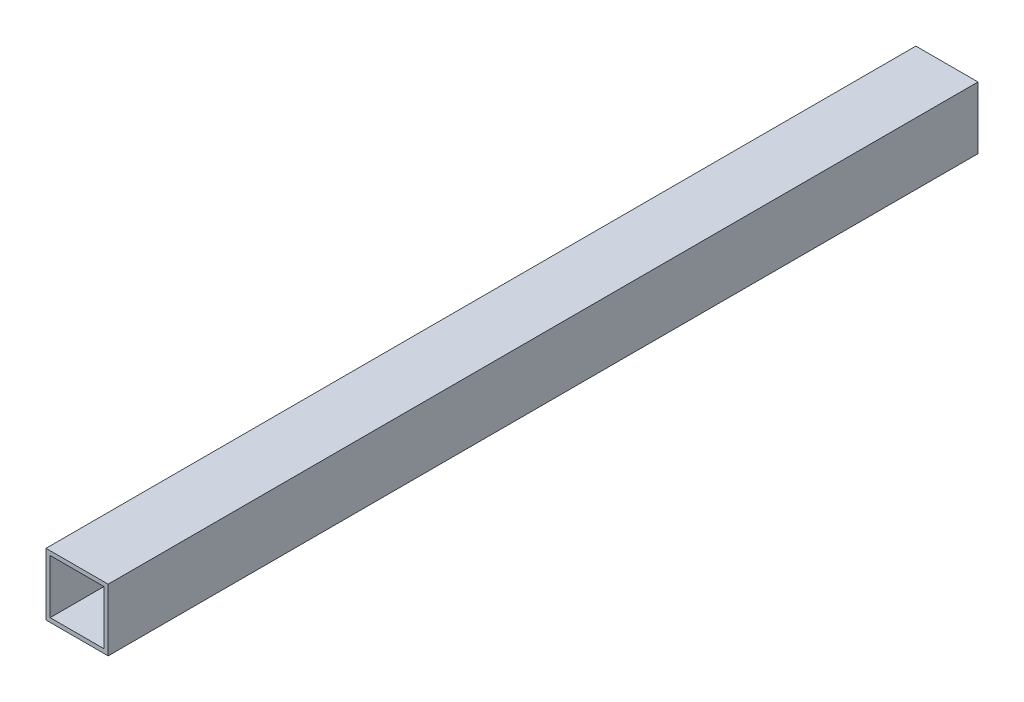
from build123d import *

# Parameters (mm, degrees)
SKETCH_1_W      = 30
SKETCH_1_H      = 30
SKETCH_1_W_2    = 26
SKETCH_1_H_2    = 26
EXTRUDE_1_DEPTH = 210


with BuildPart() as part:
    # 草图1 → 凸台-拉伸1 (new, symmetric)
    with BuildSketch(Plane.XY):
        Rectangle(SKETCH_1_W, SKETCH_1_H)
        Rectangle(SKETCH_1_W_2, SKETCH_1_H_2, mode=Mode.SUBTRACT)
    extrude(amount=EXTRUDE_1_DEPTH, both=True)


solid = part.part
